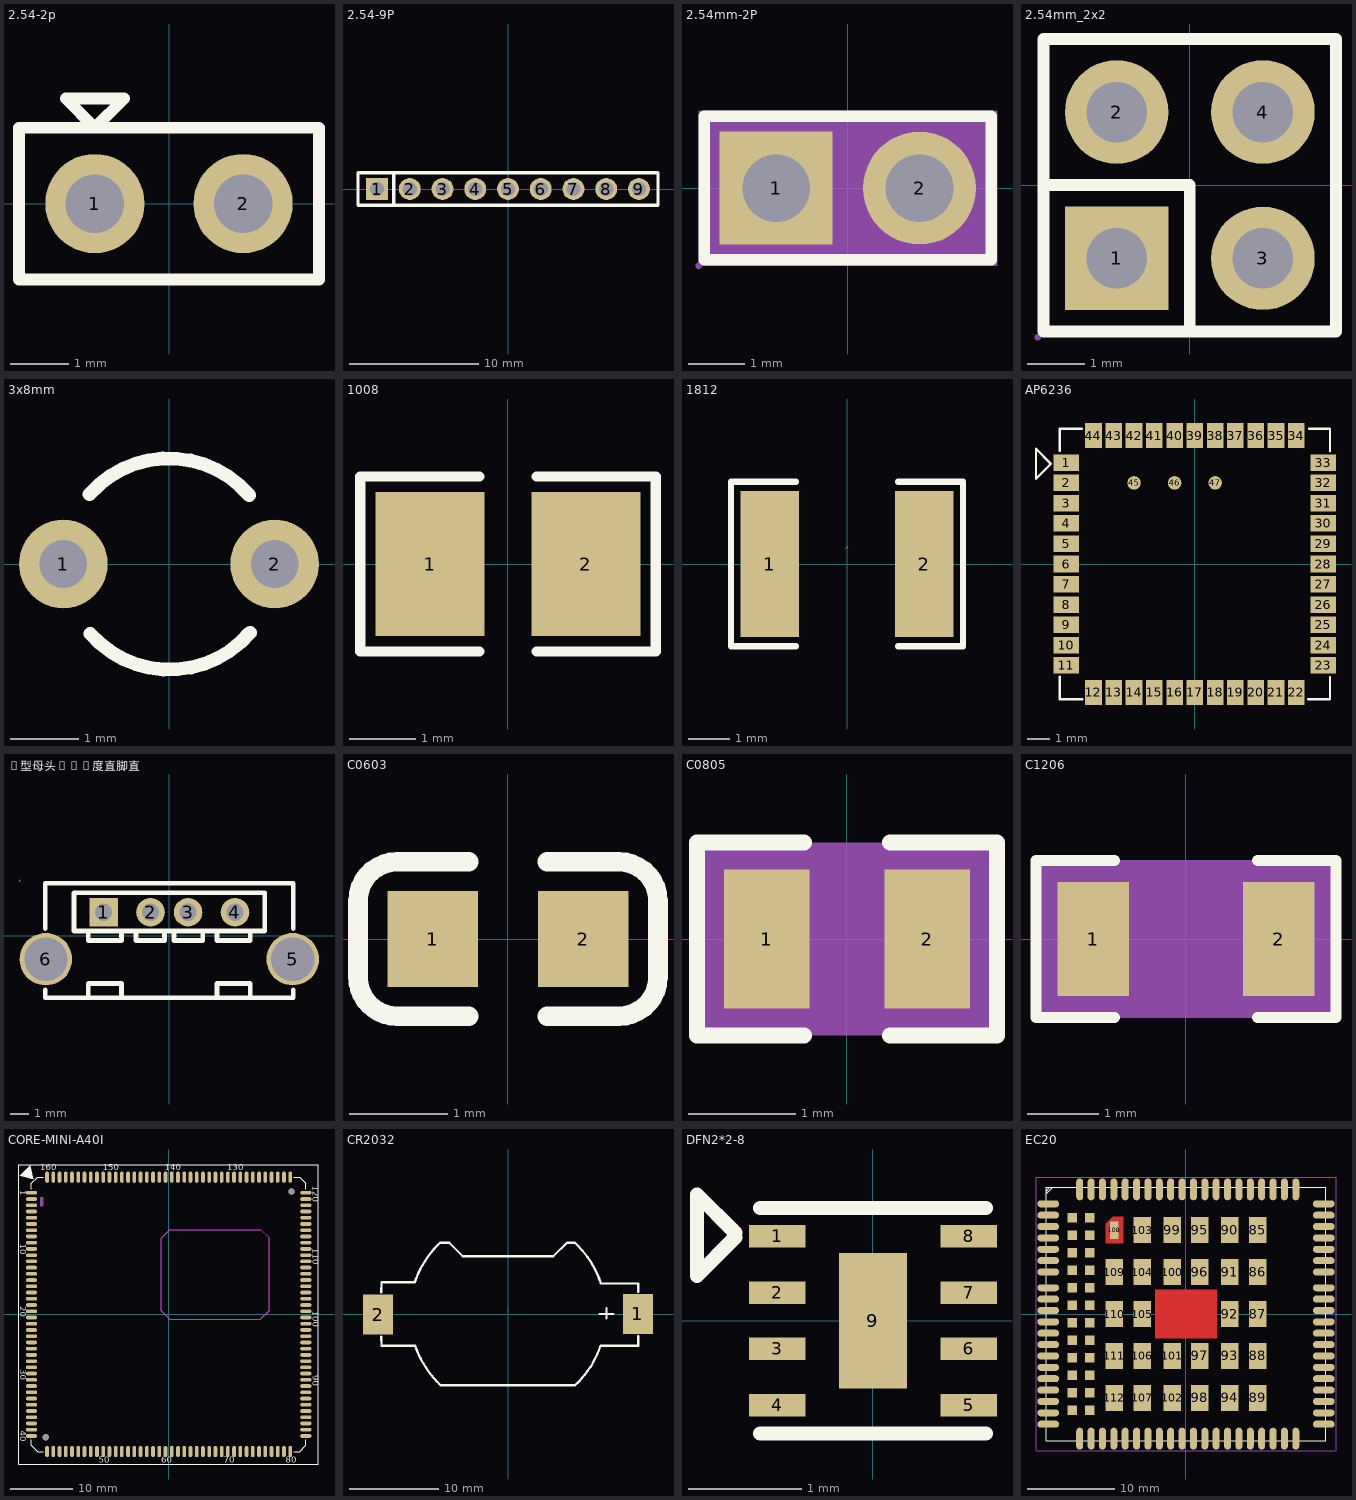
[diagram p0: the footprints below, top view; thin cyan lines are the x and y axes]
# Altium footprint library MISC84456-2.PcbLib: 53 footprints (part 1 of 4)
Each footprint in its own frame and in the unit in brackets; x right, y up, seen from the top. Pads: shape width x height; smd on the part's side, far side on the other; paste and mask are expansions set on the pad; w line width, h text height; cw(c..) or ccw(c..) is an arc to the next point about the centre after c.

## 2.54-2p [mm]
pads (2):
  round 1.7 hole 1: 1(-1.27,0) 2(1.27,0)
Top Overlay:
  lines w0.2: -2.57,0 -2.57,1.3 2.57,1.3 2.57,-1.3 -2.57,-1.3 -2.57,0.1 ; -1.77,1.8 -1.27,1.3 -0.77,1.8 -1.77,1.8
Mechanical 7:
  text "2" at 1.27,-0.254 h1.02
  text "1" at -1.27,-0.254 h1.02

## 2.54-9P [mm]
pads (9):
  rect 1.7x1.7 hole 1.1: 1(-10.16,0)
  round 1.7 hole 1.1: 2(-7.62,0) 3(-5.08,0) 4(-2.54,0) 5(0,0) 6(2.54,0) 7(5.08,0) 8(7.62,0) 9(10.16,0)
Top Overlay:
  lines w0.254: -8.866,-1.27 -8.866,1.27 ; -11.64,-1.27 -11.64,1.27 11.64,1.27 11.64,-1.27 -11.64,-1.27
Mechanical 15:
  lines w0.003: -0.025,0.451 0.025,0.502

## 2.54mm-2P [mm]
pads (2):
  rect 2x2 hole 1.2: 1(-1.27,0)
  round 2 hole 1.2: 2(1.27,0)
Top Overlay:
  lines w0.203: -2.54,-1.27 -2.54,1.27 -0.635,1.27 2.54,1.27 2.54,-1.27 -2.54,-1.27
Mechanical 4:
  region: -2.642,1.372 2.642,1.372 2.642,-1.372 -2.642,-1.372
Mechanical 5:
  circle w0.5: c1.27,0 r0.25
  circle w0.5: c-1.27,0 r0.25
Mechanical 6:
  circle w0.06: c-2.642,-1.372 r0.03
Mechanical 15:
  lines w0.003: -0.04,0.258 0.01,0.309

## 2.54mm_2x2 [mm]
pads (4):
  rect 1.8x1.8 hole 1.05: 1(-1.27,-1.27)
  round 1.8 hole 1.05: 2(-1.27,1.27) 3(1.27,-1.27) 4(1.27,1.27)
Top Overlay:
  lines w0.203: -2.54,0.002 0,0.002 0,-2.54 ; 0.212,-2.54 2.54,-2.54 ; 2.54,-2.54 2.54,2.54 -2.54,2.54 -2.54,-2.54 2.54,-2.54
Mechanical 5:
  circle w0.425: c1.27,1.27 r0.213
  circle w0.425: c1.27,-1.27 r0.213
  circle w0.425: c-1.27,1.27 r0.213
  circle w0.425: c-1.27,-1.27 r0.213
Mechanical 6:
  circle w0.06: c-2.642,-2.642 r0.03

## 3x8mm [mm]
pads (2):
  round 1.3 hole 0.7: 1(-1.55,0) 2(1.55,0)
Top Overlay:
  lines w0.2: -1.165,1.022 cw(c0,0) 1.179,1.006 ; -1.155,-1.022 ccw(c0.01,0) 1.189,-1.006

## 1008 [mm]
pads (2):
  rect 1.635x2.16 smd: 1(-1.168,0) 2(1.168,0)
Top Overlay:
  lines w0.152: -0.426,-1.309 -2.214,-1.309 -2.214,1.309 -0.426,1.309 ; 0.426,-1.309 2.214,-1.309 2.214,1.309 0.426,1.309
Top Paste:
  region: -0.315,-0.98 -0.315,-0.467 -0.415,-0.367 -0.806,-0.367 -0.906,-0.267 -0.906,0.267 -0.806,0.367 -0.415,0.367 -0.315,0.467 -0.315,0.98 -0.415,1.08 -1.885,1.08 -1.985,0.98 -1.985,-0.98 -1.885,-1.08 -0.415,-1.08
  region: 0.315,-0.98 0.315,-0.467 0.415,-0.367 0.806,-0.367 0.906,-0.267 0.906,0.267 0.806,0.367 0.415,0.367 0.315,0.467 0.315,0.98 0.415,1.08 1.885,1.08 1.985,0.98 1.985,-0.98 1.885,-1.08 0.415,-1.08

## 1812 [mm]
pads (2):
  rect 1.407x3.499 smd: 1(-1.853,0) 2(1.853,0)
Top Overlay:
  lines w0.152: -1.226,-1.978 -2.785,-1.978 -2.785,1.978 -1.226,1.978 ; 1.226,-1.978 2.785,-1.978 2.785,1.978 1.226,1.978
Top Paste:
  region: -1.15,-1.65 -1.15,-0.695 -1.25,-0.595 -1.528,-0.595 -1.628,-0.495 -1.628,0.495 -1.528,0.595 -1.25,0.595 -1.15,0.695 -1.15,1.65 -1.25,1.75 -2.457,1.75 -2.557,1.65 -2.557,-1.65 -2.457,-1.75 -1.25,-1.75
  region: 1.15,-1.65 1.15,-0.695 1.25,-0.595 1.528,-0.595 1.628,-0.495 1.628,0.495 1.528,0.595 1.25,0.595 1.15,0.695 1.15,1.65 1.25,1.75 2.457,1.75 2.557,1.65 2.557,-1.65 2.457,-1.75 1.25,-1.75
Mechanical 5:
  region: 2.275,-1.62 2.275,1.62 1.525,1.62 1.525,-1.62
  region: -2.275,-1.62 -2.275,1.62 -1.525,1.62 -1.525,-1.62
Mechanical 6:
  circle w0.06: c-2.275,-1.62 r0.03
Mechanical 15:
  lines w0.003: -0.025,0.376 0.025,0.427

## AP6236 [mm]
pads (47):
  rect 1.125x0.737 smd: 1(-5.7,4.5) 2(-5.7,3.6) 3(-5.7,2.7) 4(-5.7,1.8) 5(-5.7,0.9) 6(-5.7,0) 7(-5.7,-0.9) 8(-5.7,-1.8) 9(-5.7,-2.7) 10(-5.7,-3.6) 11(-5.7,-4.5) 23(5.7,-4.5) 24(5.7,-3.6) 25(5.7,-2.7) 26(5.7,-1.8) 27(5.7,-0.9) 28(5.7,0) 29(5.7,0.9) 30(5.7,1.8) 31(5.7,2.7) 32(5.7,3.6) 33(5.7,4.5)
  rect 0.737x1.125 smd: 12(-4.5,-5.7) 13(-3.6,-5.7) 14(-2.7,-5.7) 15(-1.8,-5.7) 16(-0.9,-5.7) 17(0,-5.7) 18(0.9,-5.7) 19(1.8,-5.7) 20(2.7,-5.7) 21(3.6,-5.7) 22(4.5,-5.7) 34(4.5,5.7) 35(3.6,5.7) 36(2.7,5.7) 37(1.8,5.7) 38(0.9,5.7) 39(0,5.7) 40(-0.9,5.7) 41(-1.8,5.7) 42(-2.7,5.7) 43(-3.6,5.7) 44(-4.5,5.7)
  round 0.6 smd: 45(-2.7,3.6) 46(-0.9,3.6) 47(0.9,3.6)
Top Overlay:
  lines w0.1: -6,-5 -6,-6 -4.99,-6 ; -6,5.01 -6,6 -5.02,6 ; 5.02,-6 6,-6 6,-5.01 ; 5.07,6 6,6 6,4.99 ; -6.38,4.44 -6.38,4.44 ; -6.38,4.44 -7.05,5.11 -7.05,3.78 -6.39,4.44 -6.38,4.44

## A型母头180度直脚直 [mm]
pads (6):
  rect 1.524x1.524 hole 0.92: 1(-3.5,1.25)
  round 1.524 hole 0.92: 2(-1,1.25) 3(1,1.25) 4(3.5,1.25)
  round 2.8 hole 2.3: 5(6.575,-1.25) 6(-6.575,-1.25)
Top Overlay:
  lines w0.254: -6.604,-2.881 -6.604,-3.302 6.604,-3.302 6.604,-3.048 6.604,-2.881 ; -6.604,0.381 -6.604,2.794 6.604,2.794 6.604,0.381 ; -5.08,0.254 5.08,0.254 5.08,2.286 -5.08,2.286 -5.08,0.254 ; -4.318,-3.302 -2.54,-3.302 -2.54,-2.54 -4.318,-2.54 -4.318,-3.302 ; -4.318,-0.254 -2.54,-0.254 -2.54,0.254 -4.318,0.254 -4.318,-0.254 ; -1.778,-0.254 -0.254,-0.254 -0.254,0.254 -1.778,0.254 -1.778,-0.254 ; 0.254,-0.254 1.778,-0.254 1.778,0.254 0.254,0.254 0.254,-0.254 ; 2.54,-3.302 4.318,-3.302 4.318,-2.54 2.54,-2.54 2.54,-3.302 ; 2.54,-0.254 4.318,-0.254 4.318,0.254 2.54,0.254 2.54,-0.254
Mechanical 5:
  circle w0.36: c-3.5,1.25 r0.18
  circle w0.36: c-1,1.25 r0.18
  circle w0.36: c1,1.25 r0.18
  circle w0.36: c3.5,1.25 r0.18
  circle w1.05: c6.575,-1.25 r0.525
  circle w1.05: c-6.575,-1.25 r0.525
Mechanical 6:
  circle w0.06: c-7.975,2.921 r0.03

## C0603 [mm]
pads (2):
  rect 0.93x0.98 smd: 1(-0.77,0) 2(0.77,0)
Top Overlay:
  lines w0.2: -0.4,-0.79 -1.135,-0.79 cw(c-1.135,-0.39) -1.535,-0.39 -1.535,0.39 cw(c-1.135,0.39) -1.135,0.79 -0.4,0.79 ; 0.4,-0.79 1.135,-0.79 ccw(c1.135,-0.39) 1.535,-0.39 1.535,0.39 ccw(c1.135,0.39) 1.135,0.79 0.4,0.79
3D body: height 0.3, standoff 0, extent -0.8,-0.4 0.8,0.4

## C0805 [mm] "C0805"
pads (2):
  rect 0.8x1.3 smd: 1(-0.75,0) 2(0.75,0)
Top Overlay:
  lines w0.15: -0.4,-0.9 -1.4,-0.9 -1.4,0.9 -0.4,0.9 ; 0.4,-0.9 1.4,-0.9 1.4,0.9 0.4,0.9
Mechanical 7:
  text "2" at 0.75,0.254 h1.02
  text "1" at -0.75,0.254 h1.02
Mechanical 8:
  region: 1.4,0.9 -1.4,0.9 -1.4,-0.9 1.4,-0.9
Mechanical 9:
  text "PZ2012U221-2R0TF" at 2.9,0.025 h1.02

## C1206 [mm] "C1206"
pads (2):
  rect 1x1.6 smd: 1(-1.299,0) 2(1.3,0)
Top Overlay:
  lines w0.15: -1,-1.1 -2.1,-1.1 -2.1,1.1 -1,1.1 ; 1,-1.1 2.1,-1.1 2.1,1.1 1,1.1
Mechanical 7:
  text "1" at -1.045,0 h1.02
  text "2" at 1.554,0 h1.02
Mechanical 8:
  region: 2.1,-1.1 2.1,1.1 -2.1,1.1 -2.1,-1.1
Mechanical 9:
  text ".Designator" at 0.825,0.325 h1.02
  text "1000pF-2KV" at 1.875,0.1 h1.02

## CORE-MINI-A40I [mm] "CORE-MINI-A40I"
pads (162):
  oval 1.8x0.6 smd: 1(-22,19.5) 2(-22,18.5) 3(-22,17.5) 4(-22,16.5) 5(-22,15.5) 6(-22,14.5) 7(-22,13.5) 8(-22,12.5) 9(-22,11.5) 10(-22,10.5) 11(-22,9.5) 12(-22,8.5) 13(-22,7.5) 14(-22,6.5) 15(-22,5.5) 16(-22,4.5) 17(-22,3.5) 18(-22,2.5) 19(-22,1.5) 20(-22,0.5) 21(-22,-0.5) 22(-22,-1.5) 23(-22,-2.5) 24(-22,-3.5) 25(-22,-4.5) 26(-22,-5.5) 27(-22,-6.5) 28(-22,-7.5) 29(-22,-8.5) 30(-22,-9.5) 31(-22,-10.5) 32(-22,-11.5) 33(-22,-12.5) 34(-22,-13.5) 35(-22,-14.5) 36(-22,-15.5) 37(-22,-16.5) 38(-22,-17.5) 39(-22,-18.5) 40(-22,-19.5) 81(22,-19.5) 82(22,-18.5) 83(22,-17.5) 84(22,-16.5) 85(22,-15.5) 86(22,-14.5) 87(22,-13.5) 88(22,-12.5) 89(22,-11.5) 90(22,-10.5) 91(22,-9.5) 92(22,-8.5) 93(22,-7.5) 94(22,-6.5) 95(22,-5.5) 96(22,-4.5) 97(22,-3.5) 98(22,-2.5) 99(22,-1.5) 100(22,-0.5) 101(22,0.5) 102(22,1.5) 103(22,2.5) 104(22,3.5) 105(22,4.5) 106(22,5.5) 107(22,6.5) 108(22,7.5) 109(22,8.5) 110(22,9.5) 111(22,10.5) 112(22,11.5) 113(22,12.5) 114(22,13.5) 115(22,14.5) 116(22,15.5) 117(22,16.5) 118(22,17.5) 119(22,18.5) 120(22,19.5)
  oval 0.6x1.8 smd: 41(-19.5,-22) 42(-18.5,-22) 43(-17.5,-22) 44(-16.5,-22) 45(-15.5,-22) 46(-14.5,-22) 47(-13.5,-22) 48(-12.5,-22) 49(-11.5,-22) 50(-10.5,-22) 51(-9.5,-22) 52(-8.5,-22) 53(-7.5,-22) 54(-6.5,-22) 55(-5.5,-22) 56(-4.5,-22) 57(-3.5,-22) 58(-2.5,-22) 59(-1.5,-22) 60(-0.5,-22) 61(0.5,-22) 62(1.5,-22) 63(2.5,-22) 64(3.5,-22) 65(4.5,-22) 66(5.5,-22) 67(6.5,-22) 68(7.5,-22) 69(8.5,-22) 70(9.5,-22) 71(10.5,-22) 72(11.5,-22) 73(12.5,-22) 74(13.5,-22) 75(14.5,-22) 76(15.5,-22) 77(16.5,-22) 78(17.5,-22) 79(18.5,-22) 80(19.5,-22) 121(19.5,22) 122(18.5,22) 123(17.5,22) 124(16.5,22) 125(15.5,22) 126(14.5,22) 127(13.5,22) 128(12.5,22) 129(11.5,22) 130(10.5,22) 131(9.5,22) 132(8.5,22) 133(7.5,22) 134(6.5,22) 135(5.5,22) 136(4.5,22) 137(3.5,22) 138(2.5,22) 139(1.5,22) 140(0.5,22) 141(-0.5,22) 142(-1.5,22) 143(-2.5,22) 144(-3.5,22) 145(-4.5,22) 146(-5.5,22) 147(-6.5,22) 148(-7.5,22) 149(-8.5,22) 150(-9.5,22) 151(-10.5,22) 152(-11.5,22) 153(-12.5,22) 154(-13.5,22) 155(-14.5,22) 156(-15.5,22) 157(-16.5,22) 158(-17.5,22) 159(-18.5,22) 160(-19.5,22)
  round 1 hole 1: " "(-19.7,-19.7) " "(19.7,19.7)
Top Overlay:
  pour cut-out: -22.4,23.7 -23.7,22.4 -23.9,22.2 -21.7,21.7 -22.2,23.9
  lines w0.15: -22,-20.1 -22,-21 -21,-22 -20.1,-22 ; -22,20.1 -22,21 -21,22 -20.1,22 ; 20.1,-22 21,-22 22,-21 22,-20.1 ; 20.1,22 21,22 22,21 22,20.1 ; -24,-24 -24,24 -19.6,24 24,24 24,-24 -24,-24
  text "150" at -10.6,23.1 h1.02
  text "140" at -0.6,23.1 h1.02
  text "130" at 9.4,23.1 h1.02
  text "120" at 23.1,20.6 h1.02
  text "110" at 23.1,10.6 h1.02
  text "100" at 23.1,0.6 h1.02
  text "90" at 23.1,-9.8 h1.02
  text "80" at 18.8,-23.8 h1.02
  text "70" at 8.8,-23.8 h1.02
  text "60" at -1.2,-23.8 h1.02
  text "50" at -11.2,-23.8 h1.02
  text "30" at -23.8,-8.8 h1.02
  text "20" at -23.8,1.3 h1.02
  text "10" at -23.8,11.3 h1.02
  text "40" at -23.8,-18.7 h1.02
  text "160" at -20.6,23.1 h1.02
  text "1" at -23.8,19.9 h1.02
Keep-Out Layer:
  lines w0.025: 14.8,13.6 16.1,12.3
  lines w0.15: -1.2,0.6 0.2,-0.8 14.7,-0.8 16.1,0.6 16.1,12.3 14.8,13.6 0.2,13.6 -1.2,12.2 -1.2,0.6
Mechanical 5:
  lines w0.025: 14.8,13.6 0.2,13.6 -1.2,12.2 -1.2,0.6 0.2,-0.8 14.7,-0.8 16.1,0.6 16.1,12.3
Mechanical 7:
  text "95" at 22,-5.094 h1.02
  text "78" at 17.5,-21.594 h1.02
  text "39" at -22,-18.094 h1.02
  text "115" at 22,15.11 h1.02
  text "38" at -22,-17.094 h1.02
  text "146" at -5.5,22.61 h1.02
  text "147" at -6.5,22.61 h1.02
  text "24" at -22,-3.094 h1.02
  text "82" at 22,-18.094 h1.02
  text "148" at -7.5,22.61 h1.02
  text "26" at -22,-5.094 h1.02
  text "27" at -22,-6.094 h1.02
  text "40" at -22,-19.094 h1.02
  text "43" at -17.5,-21.594 h1.02
  text "22" at -22,-1.094 h1.02
  text "23" at -22,-2.094 h1.02
  text "4" at -22,16.703 h1.02
  text "5" at -22,15.703 h1.02
  text "92" at 22,-8.094 h1.02
  text "91" at 22,-9.094 h1.02
  text "84" at 22,-16.094 h1.02
  text "89" at 22,-11.094 h1.02
  text "96" at 22,-4.094 h1.02
  text "87" at 22,-13.094 h1.02
  text "94" at 22,-6.094 h1.02
  text "90" at 22,-10.094 h1.02
  text "83" at 22,-17.094 h1.02
  text "88" at 22,-12.094 h1.02
  text "86" at 22,-14.094 h1.02
  text "93" at 22,-7.094 h1.02
  text "85" at 22,-15.094 h1.02
  text "149" at -8.5,22.61 h1.02
  text "10" at -22,10.906 h1.02
  text "98" at 22,-2.094 h1.02
  text "101" at 22,1.11 h1.02
  text "156" at -15.5,22.61 h1.02
  text "123" at 17.5,22.61 h1.02
  text "97" at 22,-3.094 h1.02
  text "100" at 22,0.11 h1.02
  text "143" at -2.5,22.61 h1.02
  text "6" at -22,14.703 h1.02
  text "152" at -11.5,22.61 h1.02
  text "99" at 22,-1.094 h1.02
  text "102" at 22,2.11 h1.02
  text "120" at 22,20.11 h1.02
  text "81" at 22,-19.094 h1.02
  text "50" at -10.5,-21.594 h1.02
  text "113" at 22,13.11 h1.02
  text "49" at -11.5,-21.594 h1.02
  text "144" at -3.5,22.61 h1.02
  text "48" at -12.5,-21.594 h1.02
  text "7" at -22,13.703 h1.02
  text "19" at -22,1.906 h1.02
  text "122" at 18.5,22.61 h1.02
  text "51" at -9.5,-21.594 h1.02
  text "47" at -13.5,-21.594 h1.02
  text "114" at 22,14.11 h1.02
  text "46" at -14.5,-21.594 h1.02
  text "109" at 22,9.11 h1.02
  text "112" at 22,12.11 h1.02
  text "45" at -15.5,-21.594 h1.02
  text "9" at -22,11.703 h1.02
  text "44" at -16.5,-21.594 h1.02
  text "118" at 22,18.11 h1.02
  text "8" at -22,12.703 h1.02
  text "72" at 11.5,-21.594 h1.02
  text "119" at 22,19.11 h1.02
  text "121" at 19.5,22.61 h1.02
  text "73" at 12.5,-21.594 h1.02
  text "111" at 22,11.11 h1.02
  text "117" at 22,17.11 h1.02
  text "36" at -22,-15.094 h1.02
  text "33" at -22,-12.094 h1.02
  text "110" at 22,10.11 h1.02
  text "155" at -14.5,22.61 h1.02
  text "35" at -22,-14.094 h1.02
  text "65" at 4.5,-21.594 h1.02
  text "74" at 13.5,-21.594 h1.02
  text "71" at 10.5,-21.594 h1.02
  text "20" at -22,0.906 h1.02
  text "69" at 8.5,-21.594 h1.02
  text "31" at -22,-10.094 h1.02
  text "25" at -22,-4.094 h1.02
  text "68" at 7.5,-21.594 h1.02
  text "154" at -13.5,22.61 h1.02
  text "67" at 6.5,-21.594 h1.02
  text "16" at -22,4.906 h1.02
  text "62" at 1.5,-21.594 h1.02
  text "157" at -16.5,22.61 h1.02
  text "30" at -22,-9.094 h1.02
  text "42" at -18.5,-21.594 h1.02
  text "18" at -22,2.906 h1.02
  text "70" at 9.5,-21.594 h1.02
  text "63" at 2.5,-21.594 h1.02
  text "153" at -12.5,22.61 h1.02
  text "32" at -22,-11.094 h1.02
  text "29" at -22,-8.094 h1.02
  text "64" at 3.5,-21.594 h1.02
  text "37" at -22,-16.094 h1.02
  text "28" at -22,-7.094 h1.02
  text "34" at -22,-13.094 h1.02
  text "41" at -19.5,-21.594 h1.02
  text "66" at 5.5,-21.594 h1.02
  text "17" at -22,3.906 h1.02
  text "150" at -9.5,22.61 h1.02
  text "80" at 19.5,-21.594 h1.02
  text "151" at -10.5,22.61 h1.02
  text "116" at 22,16.11 h1.02
  text "76" at 15.5,-21.594 h1.02
  text "21" at -22,-0.094 h1.02
  text "3" at -22,17.703 h1.02
  text "135" at 5.5,22.61 h1.02
  text "75" at 14.5,-21.594 h1.02
  text "79" at 18.5,-21.594 h1.02
  text "11" at -22,9.906 h1.02
  text "77" at 16.5,-21.594 h1.02
  text "2" at -22,18.703 h1.02
  text "140" at 0.5,22.61 h1.02
  text "12" at -22,8.906 h1.02
  text "145" at -4.5,22.61 h1.02
  text "139" at 1.5,22.61 h1.02
  text "13" at -22,7.906 h1.02
  text "138" at 2.5,22.61 h1.02
  text "14" at -22,6.906 h1.02
  text "134" at 6.5,22.61 h1.02
  text "141" at -0.5,22.61 h1.02
  text "142" at -1.5,22.61 h1.02
  text "137" at 3.5,22.61 h1.02
  text "129" at 11.5,22.61 h1.02
  text "130" at 10.5,22.61 h1.02
  text "124" at 16.5,22.61 h1.02
  text "127" at 13.5,22.61 h1.02
  text "132" at 8.5,22.61 h1.02
  text "131" at 9.5,22.61 h1.02
  text "128" at 12.5,22.61 h1.02
  text "125" at 15.5,22.61 h1.02
  text "126" at 14.5,22.61 h1.02
  text "133" at 7.5,22.61 h1.02
  text "136" at 4.5,22.61 h1.02
  text "54" at -6.5,-21.594 h1.02
  text "52" at -8.5,-21.594 h1.02
  text "58" at -2.5,-21.594 h1.02
  text "158" at -17.5,22.61 h1.02
  text "60" at -0.5,-21.594 h1.02
  text "105" at 22,5.11 h1.02
  text "159" at -18.5,22.61 h1.02
  text "56" at -4.5,-21.594 h1.02
  text "160" at -19.5,22.61 h1.02
  text "55" at -5.5,-21.594 h1.02
  text "1" at -22,19.703 h1.02
  text "59" at -1.5,-21.594 h1.02
  text "104" at 22,4.11 h1.02
  text "108" at 22,8.11 h1.02
  text "53" at -7.5,-21.594 h1.02
  text "103" at 22,3.11 h1.02
  text "61" at 0.5,-21.594 h1.02
  text "107" at 22,7.11 h1.02
  text "57" at -3.5,-21.594 h1.02
  text "15" at -22,5.906 h1.02
  text "106" at 22,6.11 h1.02
Mechanical 8:
  region: -20.1,18.75 -20.6,18.75 -20.6,17.3 -20.1,17.3 -20.1,17.8

## CR2032 [mm]
pads (2):
  rect 3.4x4.5 smd: 1(14.575,0.032) 2(-14.575,-0.032)
Top Overlay:
  lines w0.254: -14.224,-2.508 -14.201,-3.524 -10.85,-3.524 -10.414,-3.524 ccw(c0,0.032) -7.571,-7.954 7.52,-7.954 ; -14.224,2.445 -14.201,3.588 -10.85,3.588 -10.467,3.588 ; -10.467,3.563 cw(c0,0.032) -7.618,8.032 -6.603,8.032 -5.08,6.509 5.08,6.509 6.608,8.037 7.491,8.037 cw(c0,0.032) 10.414,3.461 14.605,3.461 14.605,2.513 ; 7.52,-7.968 ccw(c0,0.032) 10.391,-3.516 ; 10.287,0.032 11.811,0.032 ; 10.391,-3.524 11.15,-3.524 14.628,-3.524 ; 11.049,-0.476 11.049,0.667 ; 14.605,-3.524 14.605,-2.449
Mechanical 15:
  lines w0.003: -0.025,0.458 0.025,0.509

## DFN2*2-8 [mm]
pads (9):
  rect 0.5x0.2 smd: 1(-0.85,0.75) 2(-0.85,0.25) 3(-0.85,-0.25) 4(-0.85,-0.75) 5(0.85,-0.75) 6(0.85,-0.25) 7(0.85,0.25) 8(0.85,0.75)
  rect 0.6x1.2 smd: 9(0,0)
Top Overlay:
  lines w0.127: -1.22,0.74 -1.56,0.4 -1.56,1.12 -1.22,0.78 ; -1,-1 1,-1 ; -1,1 1,1

## EC20 [mm]
pads (132):
  oval 2.5x0.8 smd mask+0.05: 1(-15.75,12.6) 2(-15.75,11.3) 3(-15.75,10) 4(-15.75,8.7) 5(-15.75,7.4) 6(-15.75,6.1) 7(-15.75,4.8) 8(-15.75,0.4) 9(-15.75,-0.9) 10(-15.75,-2.2) 11(-15.75,-3.5) 12(-15.75,-4.8) 13(-15.75,-6.1) 14(-15.75,-7.4) 15(-15.75,-8.7) 16(-15.75,-10) 17(-15.75,-11.3) 18(-15.75,-12.6) 37(15.75,-12.6) 38(15.75,-11.3) 39(15.75,-10) 40(15.75,-8.7) 41(15.75,-7.4) 42(15.75,-6.1) 43(15.75,-4.8) 44(15.75,-3.5) 45(15.75,-2.2) 46(15.75,-0.9) 47(15.75,0.4) 48(15.75,4.8) 49(15.75,6.1) 50(15.75,7.4) 51(15.75,8.7) 52(15.75,10) 53(15.75,11.3) 54(15.75,12.6) 141(-15.75,3) 142(-15.75,1.7) 143(15.75,1.7) 144(15.75,3)
  oval 0.8x2.5 smd mask+0.05: 19(-9.55,-14.25) 20(-8.25,-14.25) 21(-6.95,-14.25) 22(-5.65,-14.25) 23(-4.35,-14.25) 24(-3.05,-14.25) 25(-1.75,-14.25) 26(-0.45,-14.25) 27(0.85,-14.25) 28(2.15,-14.25) 29(3.45,-14.25) 30(4.75,-14.25) 31(6.05,-14.25) 32(7.35,-14.25) 33(8.65,-14.25) 34(9.95,-14.25) 35(11.25,-14.25) 36(12.55,-14.25) 55(12.55,14.25) 56(11.25,14.25) 57(9.95,14.25) 58(8.65,14.25) 59(7.35,14.25) 60(6.05,14.25) 61(4.75,14.25) 62(3.45,14.25) 63(2.15,14.25) 64(0.85,14.25) 65(-0.45,14.25) 66(-1.75,14.25) 67(-3.05,14.25) 68(-4.35,14.25) 69(-5.65,14.25) 70(-6.95,14.25) 71(-8.25,14.25) 72(-9.55,14.25) 113(-10.85,14.25) 114(-12.15,14.25) 115(-10.85,-14.25) 116(-12.15,-14.25)
  rect 2x3 smd mask+0.05: 85(8.2,9.6) 86(8.2,4.8) 87(8.2,0) 88(8.2,-4.8) 89(8.2,-9.6) 90(5,9.6) 91(5,4.8) 92(5,0) 93(5,-4.8) 94(5,-9.6) 95(1.6,9.6) 96(1.6,4.8) 97(1.6,-4.8) 98(1.6,-9.6) 99(-1.6,9.6) 100(-1.6,4.8) 101(-1.6,-4.8) 102(-1.6,-9.6) 103(-5,9.6) 104(-5,4.8) 105(-5,0) 106(-5,-4.8) 107(-5,-9.6) 109(-8.2,4.8) 110(-8.2,0) 111(-8.2,-4.8) 112(-8.2,-9.6)
  rect 1x2 smd: 108(-8.2,9.6)
  rect 1.1x1.1 smd mask+0.05: 117(-11,11) 118(-11,9) 119(-11,7) 120(-11,5) 121(-11,3) 122(-11,1) 123(-11,-1) 124(-11,-3) 125(-11,-5) 126(-11,-7) 127(-11,-9) 128(-11,-11) 129(-13,11) 130(-13,9) 131(-13,7) 132(-13,5) 133(-13,3) 134(-13,1) 135(-13,-1) 136(-13,-3) 137(-13,-5) 138(-13,-7) 139(-13,-9) 140(-13,-11)
Top Layer:
  pour cut-out: 3.5,2.8 -3.5,2.8 -3.5,-2.8 3.5,-2.8
  region: -9.2,10.3 -8.4,11.1 -7.2,11.1 -7.2,8.1 -9.2,8.1
Top Overlay:
  lines w0.102: -16,13.75 -15.25,14.5 ; -16,14.5 -16,14.05 -15.55,14.5 -16,14.5 ; -16,14.5 -16,-14.5 16,-14.5 16,14.5 -16,14.5
Top Paste:
  region: -9.2,10.3 -8.4,11.1 -7.2,11.1 -7.2,8.1 -9.2,8.1
Top Solder:
  region: -9.25,8.05 -7.15,8.05 -7.15,11.15 -8.45,11.15 -9.25,10.35
Mechanical 1:
  lines w0.01: -17.15,-15.65 -17.15,15.65 17.15,15.65 17.15,-15.65 -17.15,-15.65